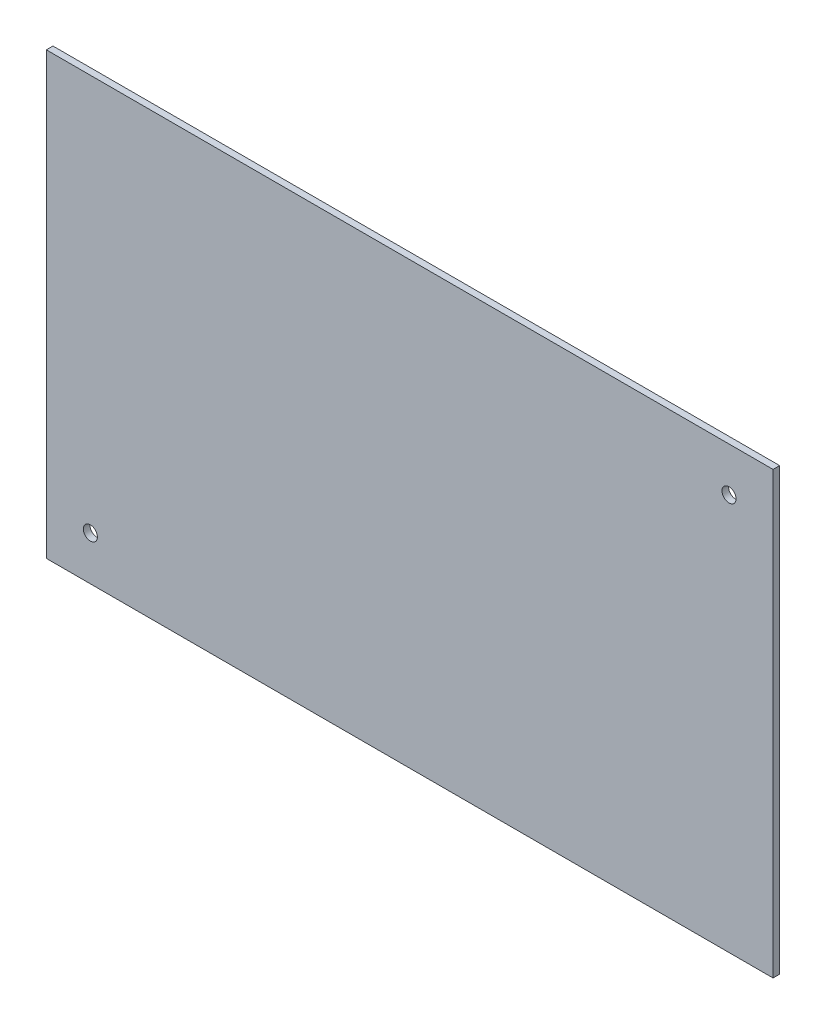
from build123d import *

# Parameters (mm, degrees)
SKETCH_1_W          = 330
SKETCH_1_H          = 200
EXTRUDE_1_DEPTH     = 1.5
SKETCH_2_R          = 3.2
CUT_EXTRUDE_1_DEPTH = 11.5


with BuildPart() as part:
    # 草图1 → 凸台-拉伸1 (new, symmetric)
    with BuildSketch(Plane.XY):
        Rectangle(SKETCH_1_W, SKETCH_1_H)
    extrude(amount=EXTRUDE_1_DEPTH, both=True)

    # 草图2 → 切除-拉伸1 (cut, symmetric)
    with BuildSketch(Plane.XY):
        with Locations((-145, -80)):
            Circle(SKETCH_2_R)
        with Locations((145, 80)):
            Circle(SKETCH_2_R)
    extrude(amount=CUT_EXTRUDE_1_DEPTH, both=True, mode=Mode.SUBTRACT)


solid = part.part
